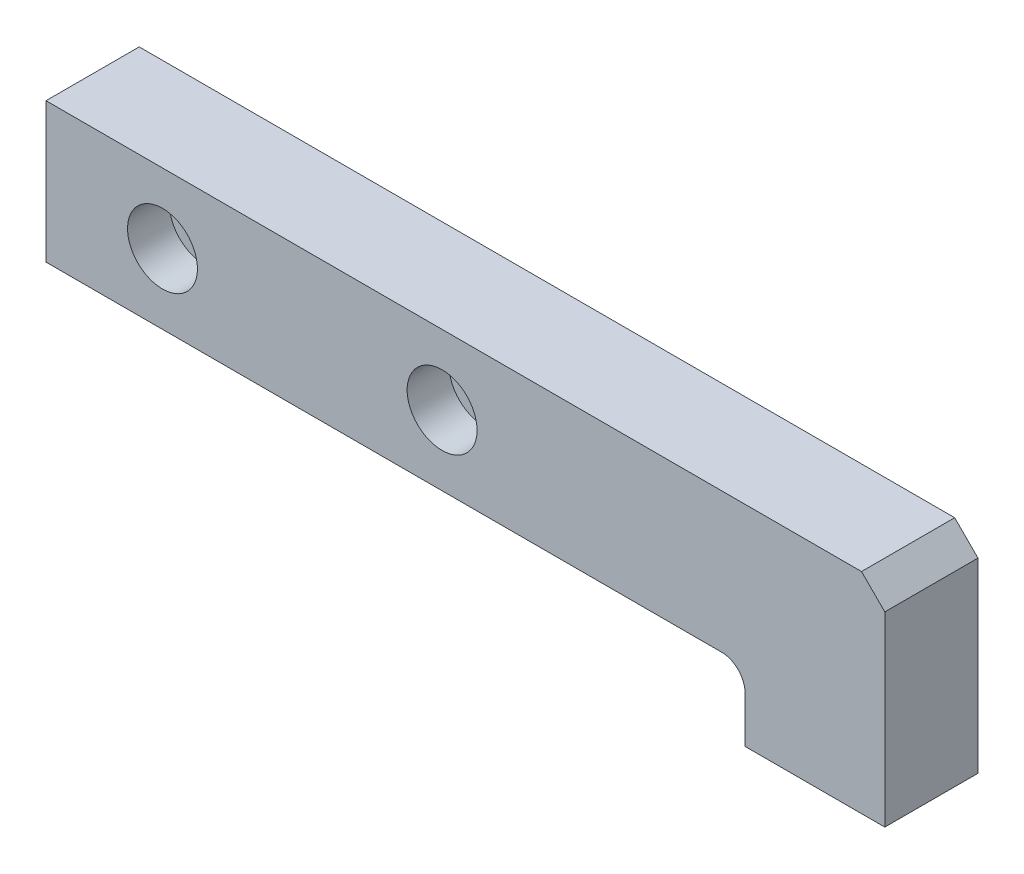
from build123d import *

# Parameters (mm, degrees)
SKETCH_1_W                = 180
SKETCH_1_H                = 30
EXTRUDE_1_DEPTH           = 20
HOLE_WIZARD_1_D           = 9
HOLE_WIZARD_1_CBORE_D     = 15
HOLE_WIZARD_1_CBORE_DEPTH = 9
SKETCH_4_W                = 30
SKETCH_4_H                = 15
EXTRUDE_2_DEPTH           = 20
FILLET_1_R                = 5
CHAMFER_1_SIZE            = 5
HOLE_WIZARD_M8_2_D        = 6.8
HOLE_WIZARD_M8_2_DEPTH    = 19.75
HOLE_WIZARD_M8_2_TIP      = 2.042926105


with BuildPart() as part:
    # 草图1 → 凸台-拉伸1 (new body)
    with BuildSketch(Plane.XY):
        Rectangle(SKETCH_1_W, SKETCH_1_H)
    extrude(amount=EXTRUDE_1_DEPTH)

    # 打孔尺寸(%根据)内六角圆柱头螺钉的类型1 (through all)
    with Locations(Plane.XY.offset(20)):
        with Locations((-65, 0), (-5, 0)):
            CounterBoreHole(HOLE_WIZARD_1_D / 2, HOLE_WIZARD_1_CBORE_D / 2, HOLE_WIZARD_1_CBORE_DEPTH)

    # 草图4 → 凸台-拉伸2 (add)
    with BuildSketch(Plane.XY.offset(20)):
        with Locations((75, -22.5)):
            Rectangle(SKETCH_4_W, SKETCH_4_H)
    extrude(amount=-EXTRUDE_2_DEPTH)

    # 圆角1
    fillet_1_edges = [part.edges().sort_by_distance(p)[0] for p in [
        (60, -15, 10),
    ]]
    fillet(fillet_1_edges, radius=FILLET_1_R)

    # 倒角1
    chamfer_1_edges = [part.edges().sort_by_distance(p)[0] for p in [
        (90, 15, 10),
    ]]
    chamfer(chamfer_1_edges, length=CHAMFER_1_SIZE)

    # M8 螺纹孔2
    with Locations(Plane(origin=(0, -30, 0), x_dir=(-1, 0, 0), z_dir=(0, -1, 0))):
        with Locations((-75, -10)):
            Hole(HOLE_WIZARD_M8_2_D / 2, depth=HOLE_WIZARD_M8_2_DEPTH)
            with Locations((0, 0, -(HOLE_WIZARD_M8_2_DEPTH + HOLE_WIZARD_M8_2_TIP / 2))):  # 118° drill point
                Cone(0, HOLE_WIZARD_M8_2_D / 2, HOLE_WIZARD_M8_2_TIP, mode=Mode.SUBTRACT)


solid = part.part
